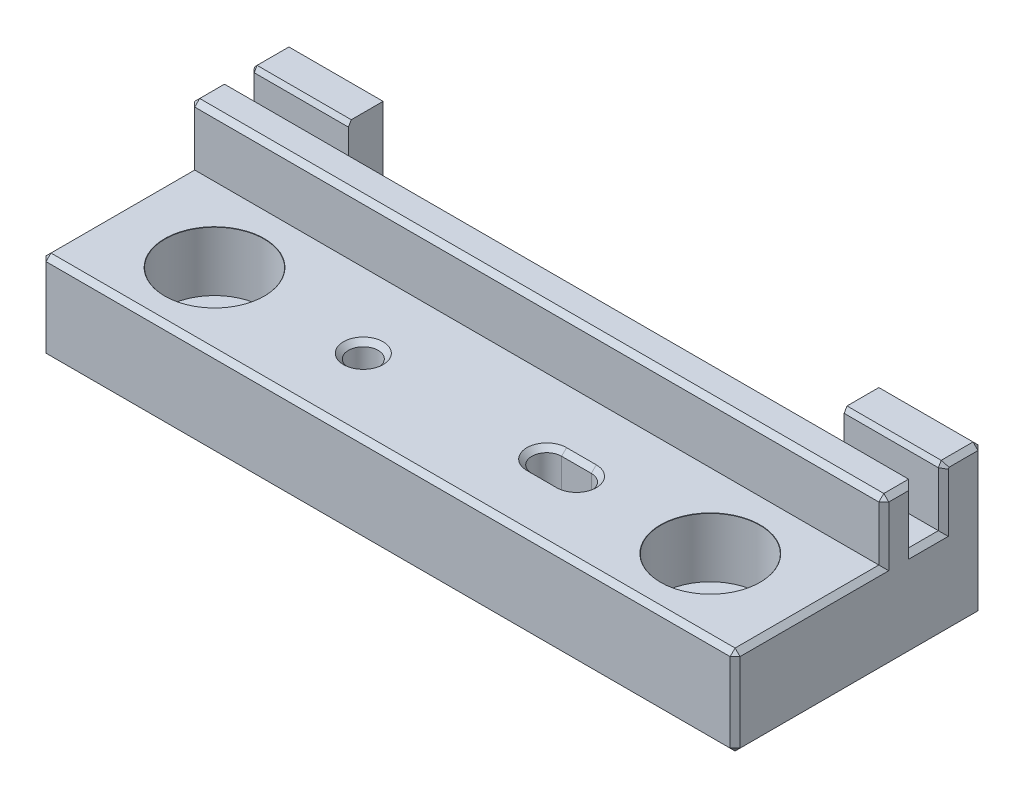
from build123d import *
from OCP.BRepFilletAPI import BRepFilletAPI_MakeChamfer

# Parameters (mm, degrees)
BOSS_EXTRUDE1_DEPTH                          = 9
SKETCH2_W                                    = 70
SKETCH2_H                                    = 3
SKETCH2_W_2                                  = 10
SKETCH2_H_2                                  = 4
BOSS_EXTRUDE2_DEPTH                          = 6
CBORE_FOR_M5_SLOTTED_CHEESE_HEAD_SCR_2_COUNT = 2
CBORE_FOR_M5_SLOTTED_CHEESE_HEAD_SCR_2_PITCH = 50
SKETCH13_R                                   = 1.5
CUT_EXTRUDE1_DEPTH                           = 75.873226189
CHAMFER3_SIZE                                = 0.5
CHAMFER3_SIZE2                               = 0.288675135
CHAMFER9_SIZE                                = 2
FILLET1_R                                    = 1
CHAMFER6_SIZE                                = 0.5
CHAMFER7_SIZE                                = 0.5
CUT_EXTRUDE2_DEPTH                           = 75.873226189
CHAMFER8_SIZE                                = 0.5


with BuildPart() as part:
    # Sketch1 → Boss-Extrude1 (new body)
    with BuildSketch(Plane(origin=(0, 0, 0), x_dir=(1, 0, 0), z_dir=(0, 1, 0))):
        Polygon((10, 21), (60, 21), (60, 25), (70, 25), (70, 0), (0, 0), (0, 25), (10, 25), align=None)
    extrude(amount=BOSS_EXTRUDE1_DEPTH)

    # Sketch2 → Boss-Extrude2 (add)
    with BuildSketch(Plane(origin=(0, 9, 0), x_dir=(1, 0, 0), z_dir=(0, 1, 0))):
        with Locations((35, 16.5)):
            Rectangle(SKETCH2_W, SKETCH2_H)
        with Locations((65, 23)):
            Rectangle(SKETCH2_W_2, SKETCH2_H_2)
        with Locations((5, 23)):
            Rectangle(SKETCH2_W_2, SKETCH2_H_2)
    extrude(amount=BOSS_EXTRUDE2_DEPTH)

    # Sketch12 → CBORE for M5 Slotted cheese head screws1 (revolve, cut)
    with BuildSketch(Plane(origin=(10, 9, -7.5), x_dir=(0, 0, 1), z_dir=(1, 0, 0))):
        Polygon((0, 0), (0, 9), (2.75, 9), (2.75, 6), (5, 6), (5, 0.025), (5.025, 0), align=None)
    cbore_for_m5_slotted_cheese_head_screws1 = revolve(axis=Axis((10, 15.35, -7.5), (0, -1, 0)), mode=Mode.SUBTRACT)

    # CBORE for M5 Slotted cheese head scr 2: CBORE for M5 Slotted cheese head screws1 ×2
    with Locations(*[(i * CBORE_FOR_M5_SLOTTED_CHEESE_HEAD_SCR_2_PITCH, 0, 0) for i in range(1, CBORE_FOR_M5_SLOTTED_CHEESE_HEAD_SCR_2_COUNT)]):
        add(cbore_for_m5_slotted_cheese_head_screws1, mode=Mode.SUBTRACT)

    # Sketch13 → Cut-Extrude1 (cut, through all)
    with BuildSketch(Plane(origin=(0, 9, 0), x_dir=(1, 0, 0), z_dir=(0, 1, 0))):
        with Locations(Location((45.000000243, 7.502702464, 0), (0, 0, 270))):
            Circle(SKETCH13_R)
        with Locations(Location((25.000000243, 7.502702464, 0), (0, 0, 270))):
            Circle(SKETCH13_R)
    extrude(amount=-CUT_EXTRUDE1_DEPTH, mode=Mode.SUBTRACT)

    # Chamfer3: one chamfer whose edges measure the first distance from different faces: ONE call of the kernel's chamfer builder (chamfer() names one face for all edges)
    chamfer3_edges_1 = [part.edges().sort_by_distance(p)[0] for p in [
        (5, 15, -21),
    ]]
    chamfer3_side_1 = [part.faces().sort_by_distance(p)[0] for p in [
        (5, 12, -21),
    ]]
    chamfer3_edges_2 = [part.edges().sort_by_distance(p)[0] for p in [
        (65, 15, -21),
    ]]
    chamfer3_side_2 = [part.faces().sort_by_distance(p)[0] for p in [
        (65, 12, -21),
    ]]
    chamfer3 = BRepFilletAPI_MakeChamfer(part.part.solid().wrapped)
    for e in chamfer3_edges_1:
        chamfer3.Add(CHAMFER3_SIZE, CHAMFER3_SIZE2, e.wrapped, chamfer3_side_1[0].wrapped)  # the first distance lies on this face
    for e in chamfer3_edges_2:
        chamfer3.Add(CHAMFER3_SIZE, CHAMFER3_SIZE2, e.wrapped, chamfer3_side_2[0].wrapped)  # the first distance lies on this face
    add(Compound.cast(chamfer3.Shape()), mode=Mode.REPLACE)

    # Chamfer9
    chamfer9_edges = [part.edges().sort_by_distance(p)[0] for p in [
        (35, 9, -21),
    ]]
    chamfer(chamfer9_edges, length=CHAMFER9_SIZE)

    # Fillet1
    fillet1_edges = [part.edges().sort_by_distance(p)[0] for p in [
        (10, 3.5, -21),
        (60, 3.5, -21),
    ]]
    fillet(fillet1_edges, radius=FILLET1_R)

    # Chamfer6
    chamfer6_edges = [part.edges().sort_by_distance(p)[0] for p in [
        (65, 0, -25),
        (70, 0, -12.5),
        (35, 0, 0),
        (0, 0, -12.5),
        (70, 9, -7.5),
        (0, 7.5, -25),
        (10, 7.5, -25),
        (60, 7.5, -25),
        (70, 7.5, -25),
        (70, 4.5, 0),
        (0, 4.5, 0),
        (0, 9, -7.5),
        (70, 9, -19.5),
        (0, 12, -18),
        (0, 12, -15),
        (70, 12, -15),
        (70, 12, -18),
        (0, 15, -16.5),
        (35, 15, -15),
        (70, 15, -16.5),
        (0, 9, -19.5),
        (0, 15, -23.144337567),
        (5, 15, -25),
        (65, 15, -25),
        (5, 0, -25),
        (70, 15, -23.144337567),
        (35, 9, 0),
        (70, 11.75, -21),
        (70, 14.75, -21.144337567),
        (0, 11.75, -21),
        (0, 14.75, -21.144337567),
    ]]
    chamfer(chamfer6_edges, length=CHAMFER6_SIZE)

    # Chamfer7
    chamfer7_edges = [part.edges().sort_by_distance(p)[0] for p in [
        (25.000000243, 0, -9.002702464),
        (25.000000243, 9, -9.002702464),
    ]]
    chamfer(chamfer7_edges, length=CHAMFER7_SIZE)

    # Sketch14 → Cut-Extrude2 (cut, through all)
    with BuildSketch(Plane(origin=(0, 9, 0), x_dir=(1, 0, 0), z_dir=(0, 1, 0))):
        with BuildLine():
            Line((43.500000243, 9.002702464), (46.500000243, 9.002702464))
            ThreePointArc((46.500000243, 9.002702464), (48.000000243, 7.502702464), (46.500000243, 6.002702464))
            Line((46.500000243, 6.002702464), (43.500000243, 6.002702464))
            ThreePointArc((43.500000243, 6.002702464), (42.000000243, 7.502702464), (43.500000243, 9.002702464))
        make_face()
    extrude(amount=-CUT_EXTRUDE2_DEPTH, mode=Mode.SUBTRACT)

    # Chamfer8
    chamfer8_edges = [part.edges().sort_by_distance(p)[0] for p in [
        (45.000000243, 0, -9.002702464),
        (45.000000243, 0, -6.002702464),
        (45.000000243, 9, -6.002702464),
        (45.000000243, 9, -9.002702464),
        (42.000000243, 9, -7.502702464),
        (48.000000243, 9, -7.502702464),
        (42.000000243, 0, -7.502702464),
        (48.000000243, 0, -7.502702464),
    ]]
    chamfer(chamfer8_edges, length=CHAMFER8_SIZE)


solid = part.part
